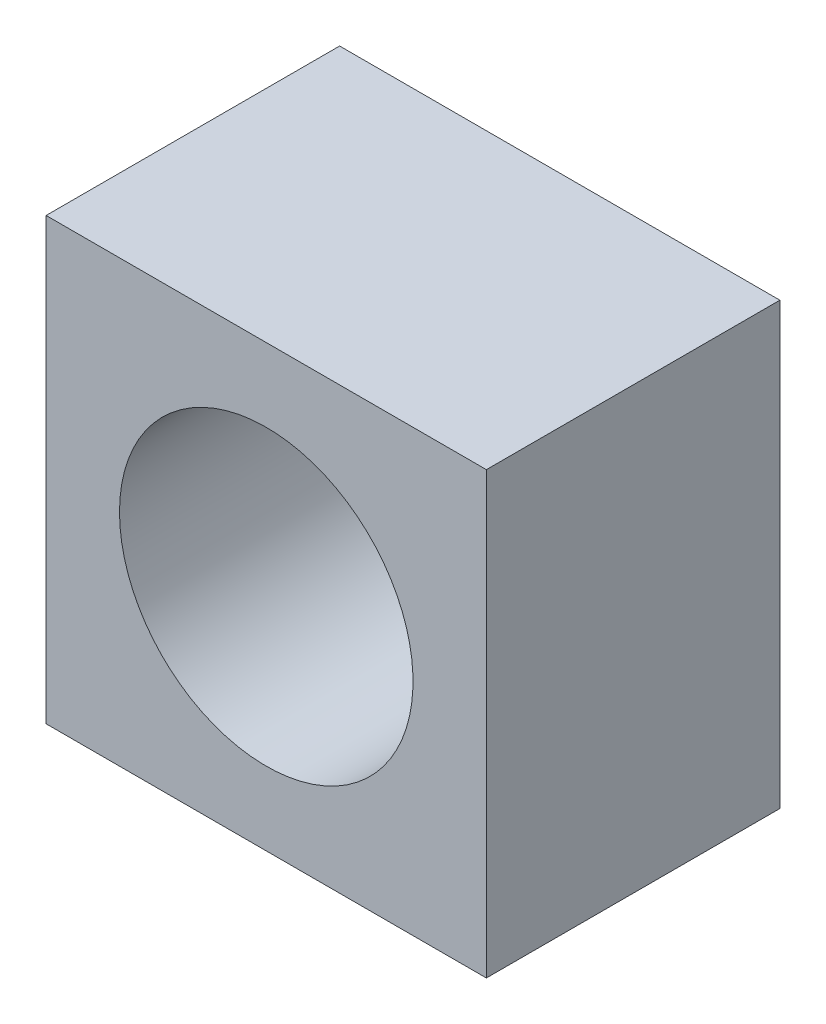
from build123d import *

# Parameters (mm, degrees)
SKETCH1_W           = 30
SKETCH1_H           = 30
SKETCH1_R           = 10
BOSS_EXTRUDE1_DEPTH = 20


with BuildPart() as part:
    # Sketch1 → Boss-Extrude1 (new body)
    with BuildSketch(Plane.XY.offset(10)):
        Rectangle(SKETCH1_W, SKETCH1_H)
        with Locations(Location((0, 0, 0), (0, 0, 180))):
            Circle(SKETCH1_R, mode=Mode.SUBTRACT)
    extrude(amount=-BOSS_EXTRUDE1_DEPTH)


solid = part.part
